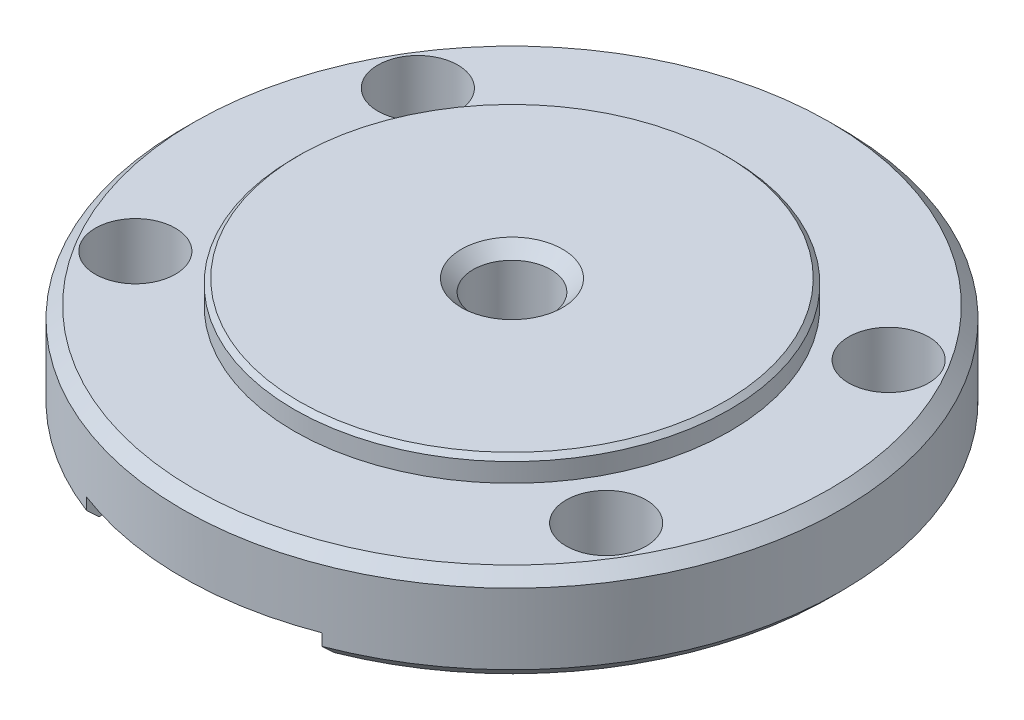
SolidWorks part; units mm, degrees
material "黑赛钢"
ref_plane "Front Plane" through (0, 0, 0) normal (0, 0, 1) x (1, 0, 0)
ref_plane "Top Plane" through (0, 0, 0) normal (0, 1, 0) x (1, 0, 0)
ref_plane "Right Plane" through (0, 0, 0) normal (1, 0, 0) x (0, 0, -1)
sketch "Sketch1" plane through (0, 0, 0) normal (0, 0, 1) x (1, 0, 0)
  line L0 (0, 0) -> (0, 15.9797) construction
  line L1 (0, 0) -> (14, 0)
  line L2 (14, 0) -> (14, 5)
  line L3 (14, 5) -> (0, 5)
  line L8 (0, 5) -> (0, 0)
  dimension "D1" = 14
  dimension "D2" = 5
revolve "Revolve1" add sketch "Sketch1" angle 360 about L0
sketch "Sketch3" plane through (0, 5, 0) normal (0, 1, 0) x (1, 0, 0)
  circle A0 centre (0, 0) radius 9.25
  dimension "D1" = 18.5
extrude "Cut-Extrude2" cut sketch "Sketch3" against normal blind 1 flip side to cut
hole_wizard "M3 Clearance Hole1" positions "Sketch5" profile "Sketch4" hole size "M3" standard "GB" end condition up to next
sketch "Sketch5" plane through (0, 0, 0) normal (0, -1, 0) x (-1, 0, 0)
  line L1 (-10, -6) -> (10, -6) construction
  line L2 (-10, -6) -> (-10, 6) construction
  line L3 (-10, 6) -> (10, 6) construction
  line L4 (10, -6) -> (10, 6) construction
  line L5 (-10, -6) -> (10, 6) construction
  line L6 (-10, 6) -> (10, -6) construction
  point P0 (10, -6)
  point P2 (10, 6)
  point P4 (-10, -6)
  point P6 (-10, 6)
  dimension "D1" = 20
  dimension "D2" = 12
sketch "Sketch4" plane through (-10, 0, 6) normal (1, 0, 0) x (0, 0, -1)
  line L0 (0, 0) -> (0, 4)
  line L1 (0, 4) -> (1.7, 4)
  line L2 (1.7, 4) -> (1.7, 0)
  line L5 (1.7, 0) -> (0, 0)
  line L11 (0, -6.35) -> (0, 107.95) construction
  dimension "通孔孔直径" = 3.4
  dimension "通孔孔深度" = 4
sketch "Sketch6" plane through (0, 0, 0) normal (0, -1, 0) x (1, 0, 0)
  line L1 (5, 15.7142) -> (-5, 15.7142)
  line L2 (5, 15.7142) -> (5, -15.7142)
  line L3 (5, -15.7142) -> (-5, -15.7142)
  line L4 (-5, 15.7142) -> (-5, -15.7142)
  line L5 (5, 15.7142) -> (-5, -15.7142) construction
  line L6 (5, -15.7142) -> (-5, 15.7142) construction
  point P0 (0, 0)
  dimension "D1" = 10
extrude "Cut-Extrude3" cut sketch "Sketch6" against normal blind 1
hole_wizard "M4 Tapped Hole1" positions "Sketch9" profile "Sketch8" tap size "M4" standard "GB" end condition up to next
sketch "Sketch9" plane through (0, 1, 0) normal (0, -1, 0) x (-1, 0, 0)
  point P0 (0, 0)
sketch "Sketch8" plane through (0, 1, 0) normal (1, 0, 0) x (0, 0, -1)
  line L0 (0, 0) -> (0, 4)
  line L1 (0, 4) -> (1.65, 4)
  line L2 (1.65, 4) -> (1.65, 0)
  line L5 (1.65, 0) -> (0, 0)
  line L11 (0, -6.35) -> (0, 107.95) construction
  dimension "通孔螺纹孔钻头直径" = 3.3
  dimension "通孔螺纹孔钻头深度" = 4
cosmetic thread "Hole Thread1" parameters "D2"=4
chamfer "Chamfer1" distance 0.5 angle 45 5 edges at (0, 4, 14) (14, 0, 0) (-14, 0, 0) (0, 1, -1.65) (0, 5, 1.65)
chamfer "Chamfer2" distance 0.2 angle 45 1 edges at (0, 5, 9.25)
